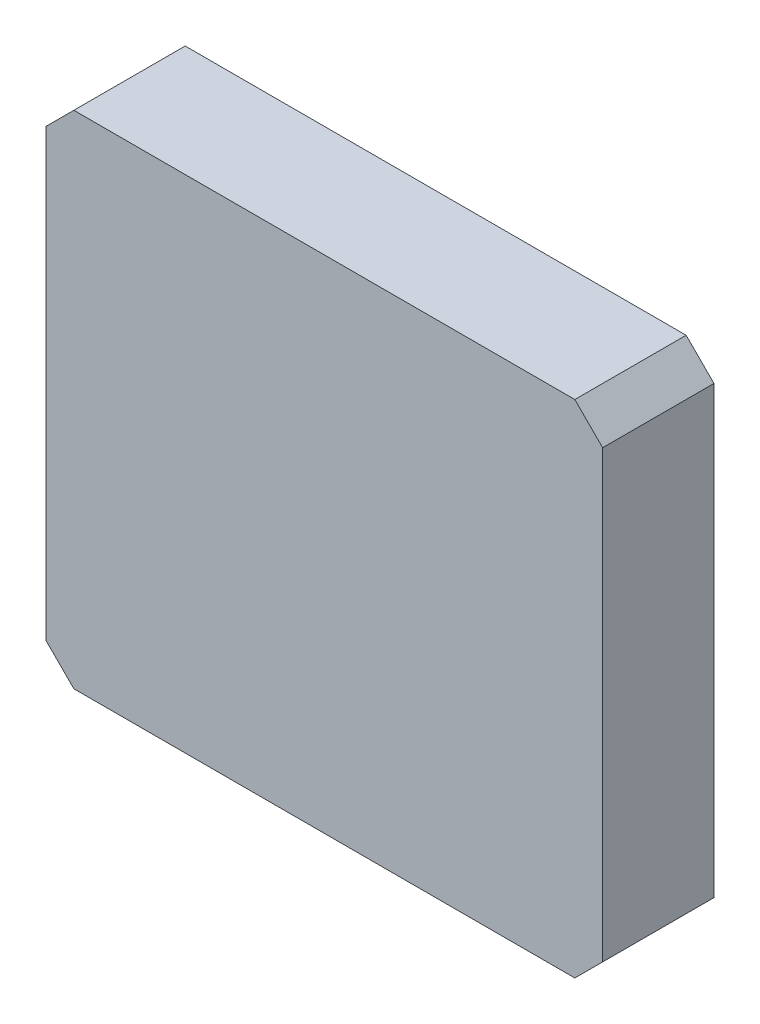
SolidWorks part; units mm, degrees
material "Q235-A"
ref_plane "Front Plane" through (0, 0, 0) normal (0, 0, 1) x (1, 0, 0)
ref_plane "Top Plane" through (0, 0, 0) normal (0, 1, 0) x (1, 0, 0)
ref_plane "Right Plane" through (0, 0, 0) normal (1, 0, 0) x (0, 0, -1)
sketch "Sketch1" plane through (0, 0, 0) normal (0, 0, 1) x (1, 0, 0)
  line L1 (-46.6158, 47.2581) -> (53.3842, 47.2581)
  line L2 (-46.6158, 47.2581) -> (-46.6158, -42.7419)
  line L3 (-46.6158, -42.7419) -> (53.3842, -42.7419)
  line L4 (53.3842, 47.2581) -> (53.3842, -42.7419)
  dimension "D1" = 100
  dimension "D2" = 90
extrude "Boss-Extrude1" add sketch "Sketch1" along normal blind 20
chamfer "Chamfer1" distance 5 angle 45 4 edges at (53.3842, -42.7419, 10) (-46.6158, -42.7419, 10) (-46.6158, 47.2581, 10) (53.3842, 47.2581, 10)
